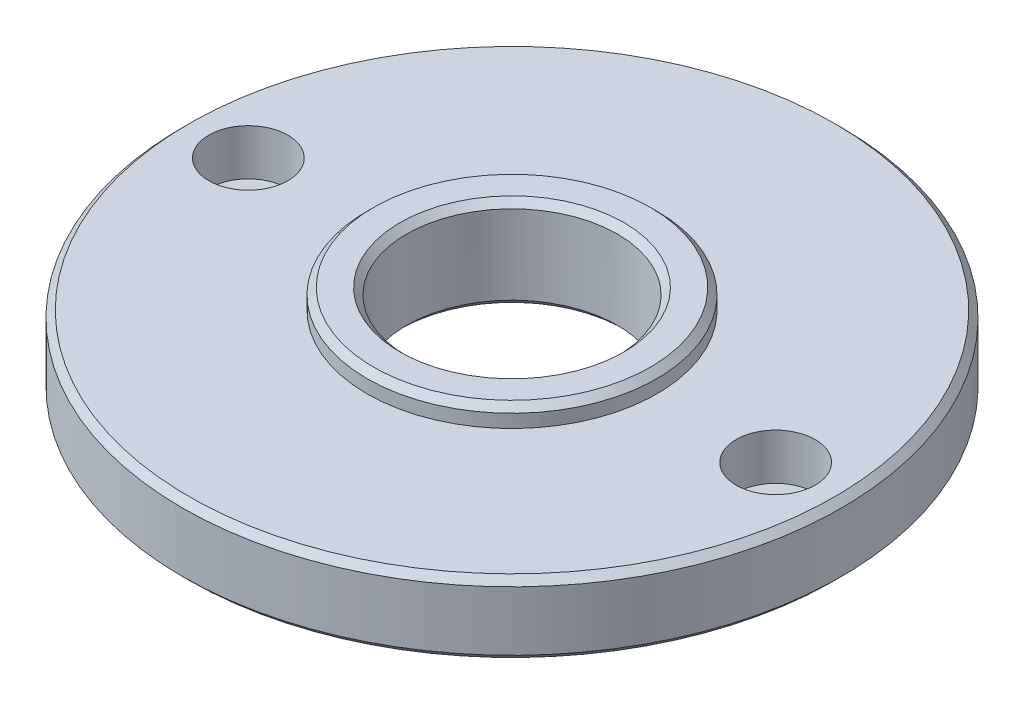
SolidWorks part; units mm, degrees
material "6061 合金"
ref_plane "Front Plane" through (0, 0, 0) normal (0, 0, 1) x (1, 0, 0)
ref_plane "Top Plane" through (0, 0, 0) normal (0, 1, 0) x (1, 0, 0)
ref_plane "Right Plane" through (0, 0, 0) normal (1, 0, 0) x (0, 0, -1)
sketch "Sketch1" plane through (0, 0, 0) normal (0, 0, 1) x (1, 0, 0)
  line L0 (0, 21.4583) -> (0, 0) construction
  line L4 (8, 0) -> (25, 0)
  line L5 (25, 0) -> (25, 5.5)
  line L6 (25, 5.5) -> (11, 5.5)
  line L7 (11, 7) -> (11, 5.5)
  line L8 (11, 7) -> (8, 7)
  line L9 (8, 7) -> (8, 0)
  dimension "D2" = 25
  dimension "D4" = 5.5
  dimension "D5" = 11
  dimension "D6" = 8
  dimension "D8" = 1.5
revolve "Revolve1" add sketch "Sketch1" angle 360 about L0
sketch "Sketch2" plane through (0, 5.5, 0) normal (0, -1, 0) x (1, 0, 0)
  line L0 (0, 0) -> (0, -17.8907) construction
  circle A0 centre (0, 0) radius 20 construction
  circle A1 centre (-20, 0) radius 1.75
  circle A2 centre (20, 0) radius 1.75
  dimension "D1" = 40
  dimension "D2" = 3.5
hole_wizard "CBORE for M3 Hex Head Bolt1" positions "3DSketch1" profile "Sketch3" counterbore size "M3" standard "GB" end condition up to next
sketch3d "3DSketch1"
  point P0 (-20, 5.5, 0)
  point P3 (20, 5.5, 0)
sketch "Sketch3" plane through (-20, 5.5, 0) normal (1, 0, 0) x (0, 0, 1)
  line L0 (0, 0) -> (0, 5.5)
  line L1 (0, 5.5) -> (1.75, 5.5)
  line L3 (1.75, 5.5) -> (1.75, 3.5)
  line L4 (1.75, 3.5) -> (3, 3.5)
  line L5 (3, 3.5) -> (3, 0)
  line L7 (3, 0) -> (0, 0)
  line L11 (0, -6.35) -> (0, 107.95) construction
  dimension "通孔孔直径" = 3.5
  dimension "通孔孔深度" = 5.5
  dimension "柱形沉头孔直径" = 6
  dimension "柱形沉头孔深度" = 3.5
chamfer "Chamfer1" distance 0.5 angle 45 5 edges at (0, 0, 25) (0, 5.5, 25) (0, 7, 11) (0, 7, 8) (0, 0, 8)
